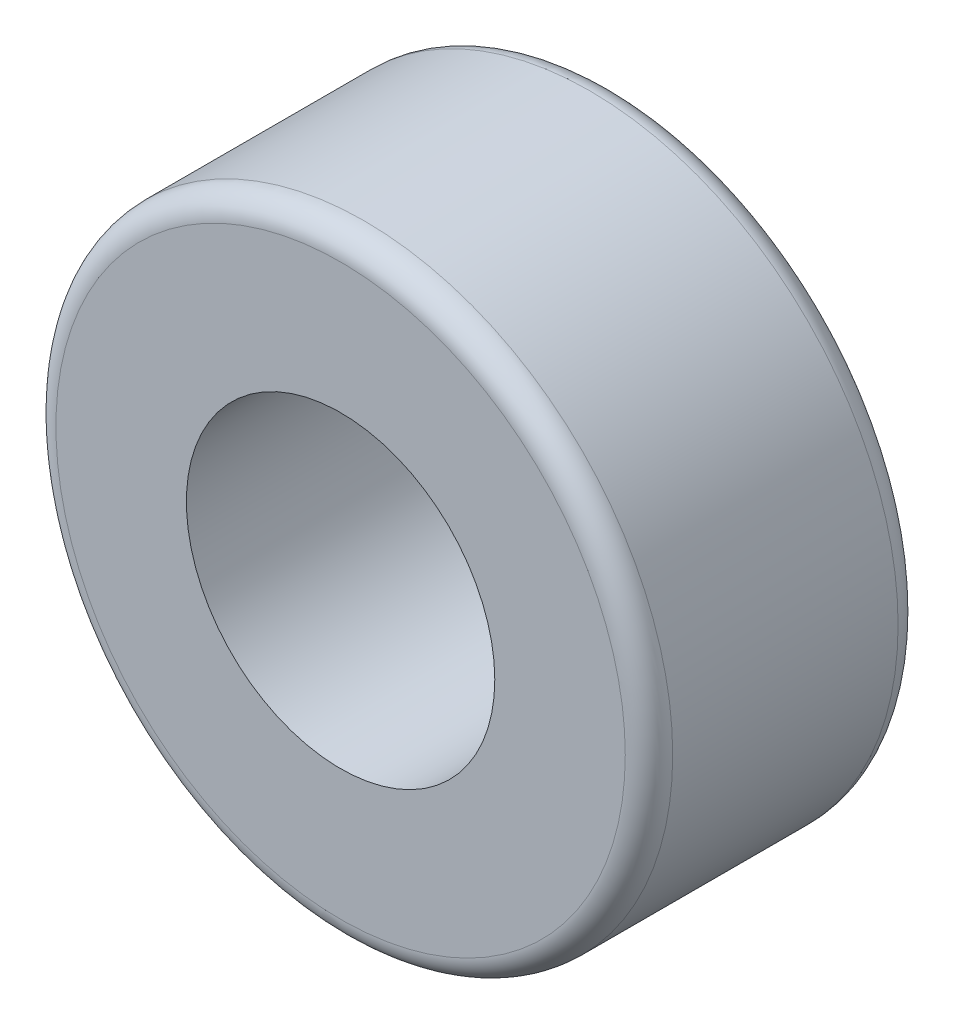
from build123d import *

# Parameters (mm, degrees)
SKETCH_1_R      = 13
SKETCH_1_R_2    = 6.5
EXTRUDE_1_DEPTH = 11.5
FILLET_1_R      = 1


with BuildPart() as part:
    # 草图1 → 凸台-拉伸1 (new body)
    with BuildSketch(Plane.XY):
        Circle(SKETCH_1_R)
        Circle(SKETCH_1_R_2, mode=Mode.SUBTRACT)
    extrude(amount=EXTRUDE_1_DEPTH)

    # 圆角1
    fillet_1_edges = [part.edges().sort_by_distance(p)[0] for p in [
        (-13, 0, 0),
        (-13, 0, 11.5),
    ]]
    fillet(fillet_1_edges, radius=FILLET_1_R)


solid = part.part
